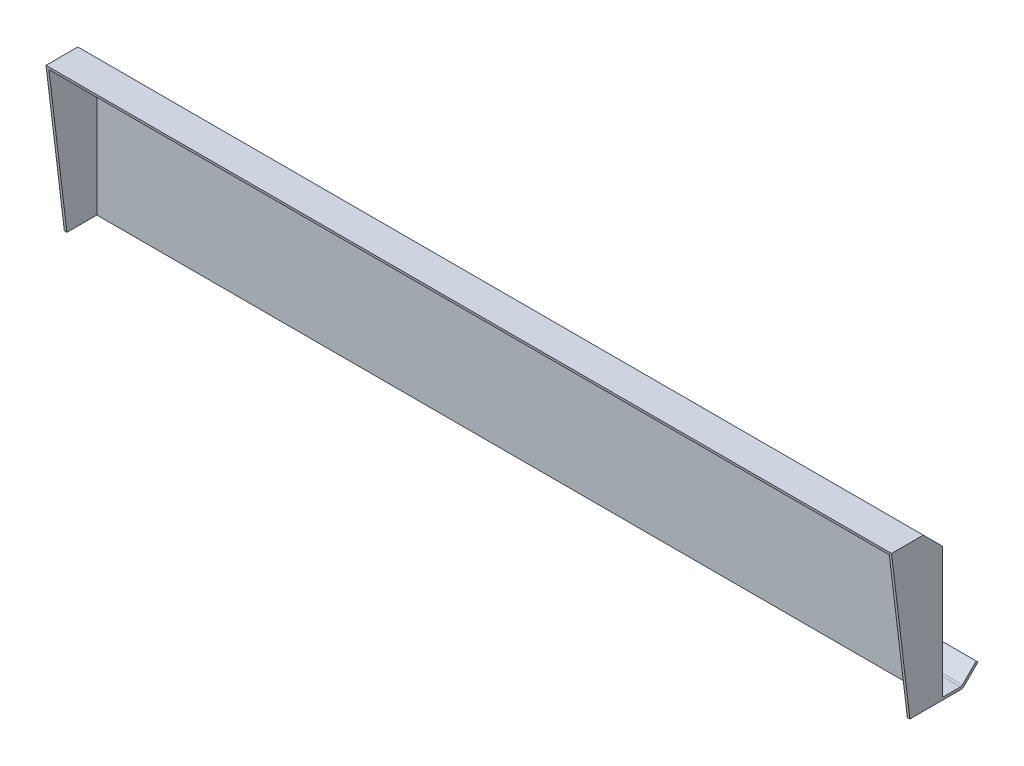
from build123d import *

# Parameters (mm, degrees)
BOSS_EXTRUDE1_DEPTH = 332.5
CHAMFER1_SIZE       = 15
SHELL1_T            = -2
SKETCH7_W           = 661
SKETCH7_H           = 23.794174757
CUT_EXTRUDE1_DEPTH  = 356.077808374
BOSS_EXTRUDE2_DEPTH = 665


with BuildPart() as part:
    # Sketch1 → Boss-Extrude1 (new, symmetric)
    with BuildSketch(Plane(origin=(0, 0, 0), x_dir=(0, 0, -1), z_dir=(1, 0, 0))):
        Polygon((0, 0), (40, 0), (40, -120), (14.446601942, -120), align=None)
    extrude(amount=BOSS_EXTRUDE1_DEPTH, both=True)

    # Chamfer1
    chamfer1_edges = [part.edges().sort_by_distance(p)[0] for p in [
        (0, 0, -40),
    ]]
    chamfer(chamfer1_edges, length=CHAMFER1_SIZE)

    # Shell1
    shell1_openings = [part.faces().sort_by_distance(p)[0] for p in [
        (0, -60, -7.223300971),
    ]]
    offset(amount=SHELL1_T, openings=shell1_openings, kind=Kind.INTERSECTION)

    # Sketch7 → Cut-Extrude1 (cut, through all)
    with BuildSketch(Plane(origin=(0, -118, 0), x_dir=(1, 0, 0), z_dir=(0, 1, 0))):
        with Locations((0, 26.102912621)):
            Rectangle(SKETCH7_W, SKETCH7_H)
    extrude(amount=-CUT_EXTRUDE1_DEPTH, mode=Mode.SUBTRACT)

    # Sketch8 → Boss-Extrude2 (add)
    with BuildSketch(Plane(origin=(332.5, 0, 0), x_dir=(0, 0, -1), z_dir=(1, 0, 0))):
        with BuildLine():
            Line((40, -120), (55.171572875, -120))
            ThreePointArc((55.171572875, -120), (55.93693974, -119.847759065), (56.585786438, -119.414213562))
            Line((56.585786438, -119.414213562), (68.02081528, -107.97918472))
            Line((68.02081528, -107.97918472), (66.606601718, -106.564971157))
            Line((66.606601718, -106.564971157), (55.757359313, -117.414213562))
            ThreePointArc((55.757359313, -117.414213562), (55.108512615, -117.847759065), (54.343145751, -118))
            Line((54.343145751, -118), (40, -118))
            Line((40, -118), (40, -120))
        make_face()
    extrude(amount=-BOSS_EXTRUDE2_DEPTH)


solid = part.part
